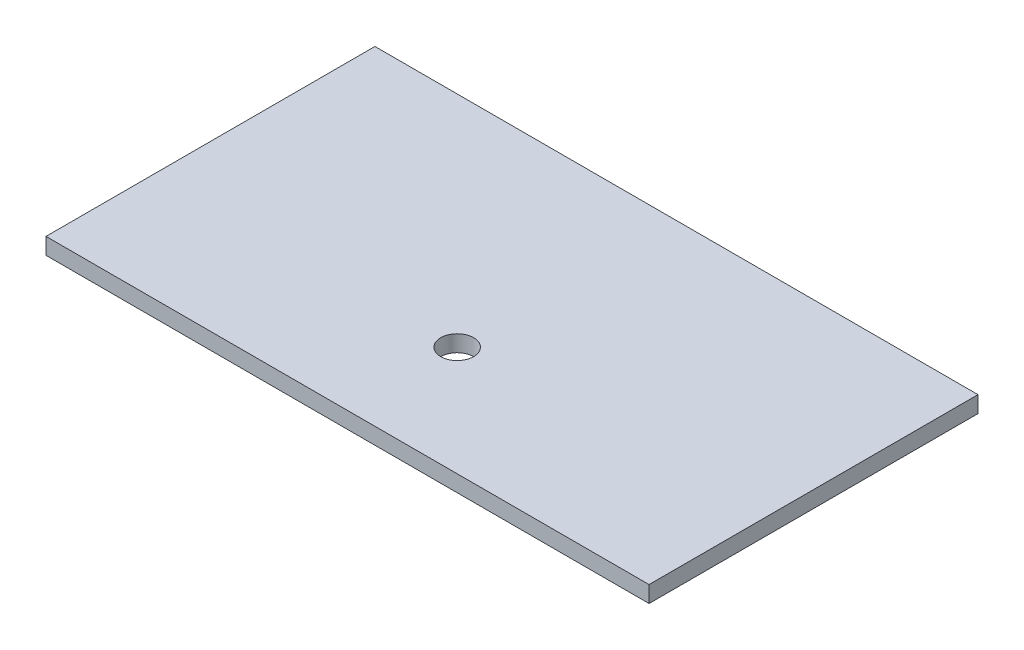
SolidWorks part; units mm, degrees
ref_plane "Front Plane" through (0, 0, 0) normal (0, 0, 1) x (1, 0, 0)
ref_plane "Top Plane" through (0, 0, 0) normal (0, 1, 0) x (1, 0, 0)
ref_plane "Right Plane" through (0, 0, 0) normal (1, 0, 0) x (0, 0, -1)
other "Configuration Table"
sketch "Sketch1" plane through (0, 0, 0) normal (0, 1, 0) x (1, 0, 0)
  line L1 (-55, -30) -> (55, -30)
  line L2 (-55, -30) -> (-55, 30)
  line L3 (-55, 30) -> (55, 30)
  line L4 (55, -30) -> (55, 30)
  line L5 (0, 30) -> (0, -30) construction
  line L6 (-55, 0) -> (55, 0) construction
  circle A0 centre (0, -10) radius 3
  point P0 (0, 0)
  dimension "D3" = 20
  dimension "D4" = 6
  dimension "D1" = 110
  dimension "D2" = 60
extrude "Boss-Extrude1" add sketch "Sketch1" along normal blind 3
